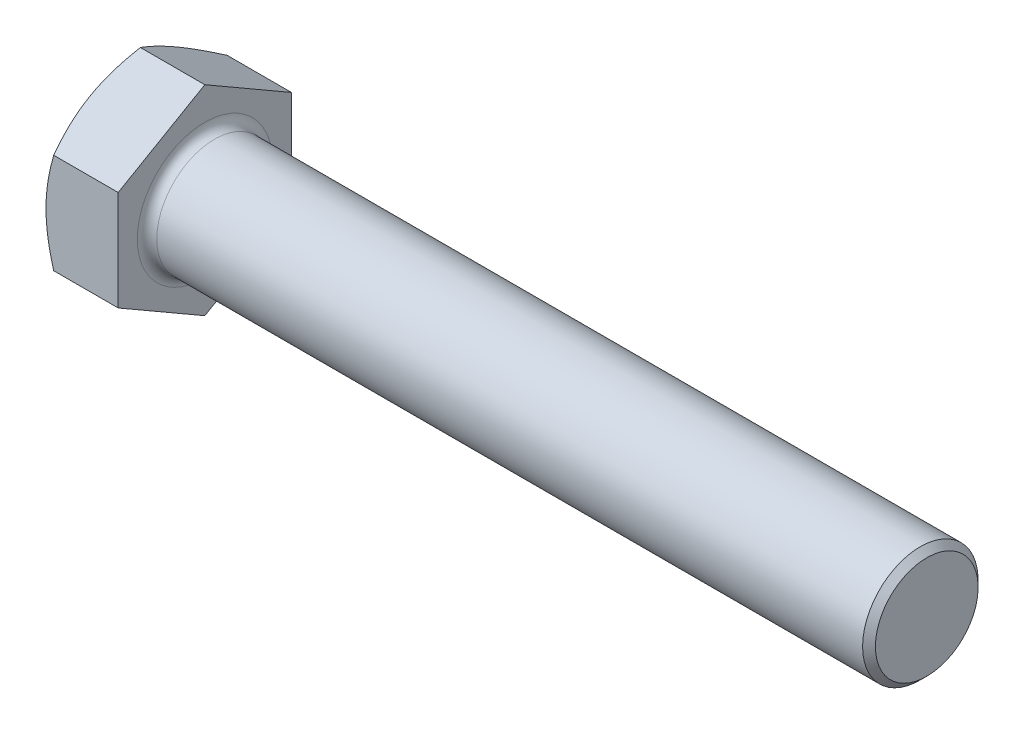
from build123d import *

# Parameters (mm, degrees)
BOSS_EXTRUDE1_DEPTH = 10
SKETCH4_R           = 26.17
SKETCH4_R_2         = 12
CUT_EXTRUDE1_DEPTH  = 1.25
CUT_EXTRUDE1_DRAFT  = -60
CHAMFER2_SIZE       = 0.888888889


with BuildPart() as part:
    # Sketch3 → Boss-Extrude1 (new body)
    with BuildSketch(Plane(origin=(0, 0, 0), x_dir=(0, 0, -1), z_dir=(1, 0, 0))):
        Polygon((12, 6.92820323), (0, 13.856406461), (-12, 6.92820323), (-12, -6.92820323), (0, -13.856406461), (12, -6.92820323), align=None)
    extrude(amount=BOSS_EXTRUDE1_DEPTH)


with BuildPart() as cut_extrude1_tool:
    # Sketch4 → Cut-Extrude1 (with draft: the straight prism first)
    with BuildSketch(Plane.ZY):
        Circle(SKETCH4_R)
        Circle(SKETCH4_R_2, mode=Mode.SUBTRACT)
    extrude(amount=-CUT_EXTRUDE1_DEPTH)
    # Cut-Extrude1: the draft: its side faces are tilted about the plane it starts from
    cut_extrude1_sides = [cut_extrude1_tool.faces().sort_by_distance(p)[0] for p in [
        (0.625, 0, -26.17),
        (0.625, 0, -12),
    ]]
    draft(cut_extrude1_sides, Plane.ZY, CUT_EXTRUDE1_DRAFT)


with BuildPart() as part_1:
    add(part.part)

    # Cut-Extrude1: cut by cut_extrude1_tool
    add(cut_extrude1_tool.part, mode=Mode.SUBTRACT)

    # Sketch5 → Revolve1 (revolve)
    with BuildSketch(Plane.XY, mode=Mode.PRIVATE) as revolve1_sk:
        with BuildLine():
            Line((11.35, 8), (110, 8))
            Line((110, 8), (110, 0))
            Line((110, 0), (10, 0))
            Line((10, 0), (10, 9.35))
            ThreePointArc((10, 9.35), (10.395405845, 8.395405845), (11.35, 8))
        make_face()
    revolve(revolve1_sk.sketch.rotate(Axis((10, 0, 0), (1, 0, 0)), 90), axis=Axis((10, 0, 0), (1, 0, 0)))

    # Chamfer2
    chamfer2_edges = [part_1.edges().sort_by_distance(p)[0] for p in [
        (110, 0, -8),
    ]]
    chamfer(chamfer2_edges, length=CHAMFER2_SIZE)


solid = part_1.part
